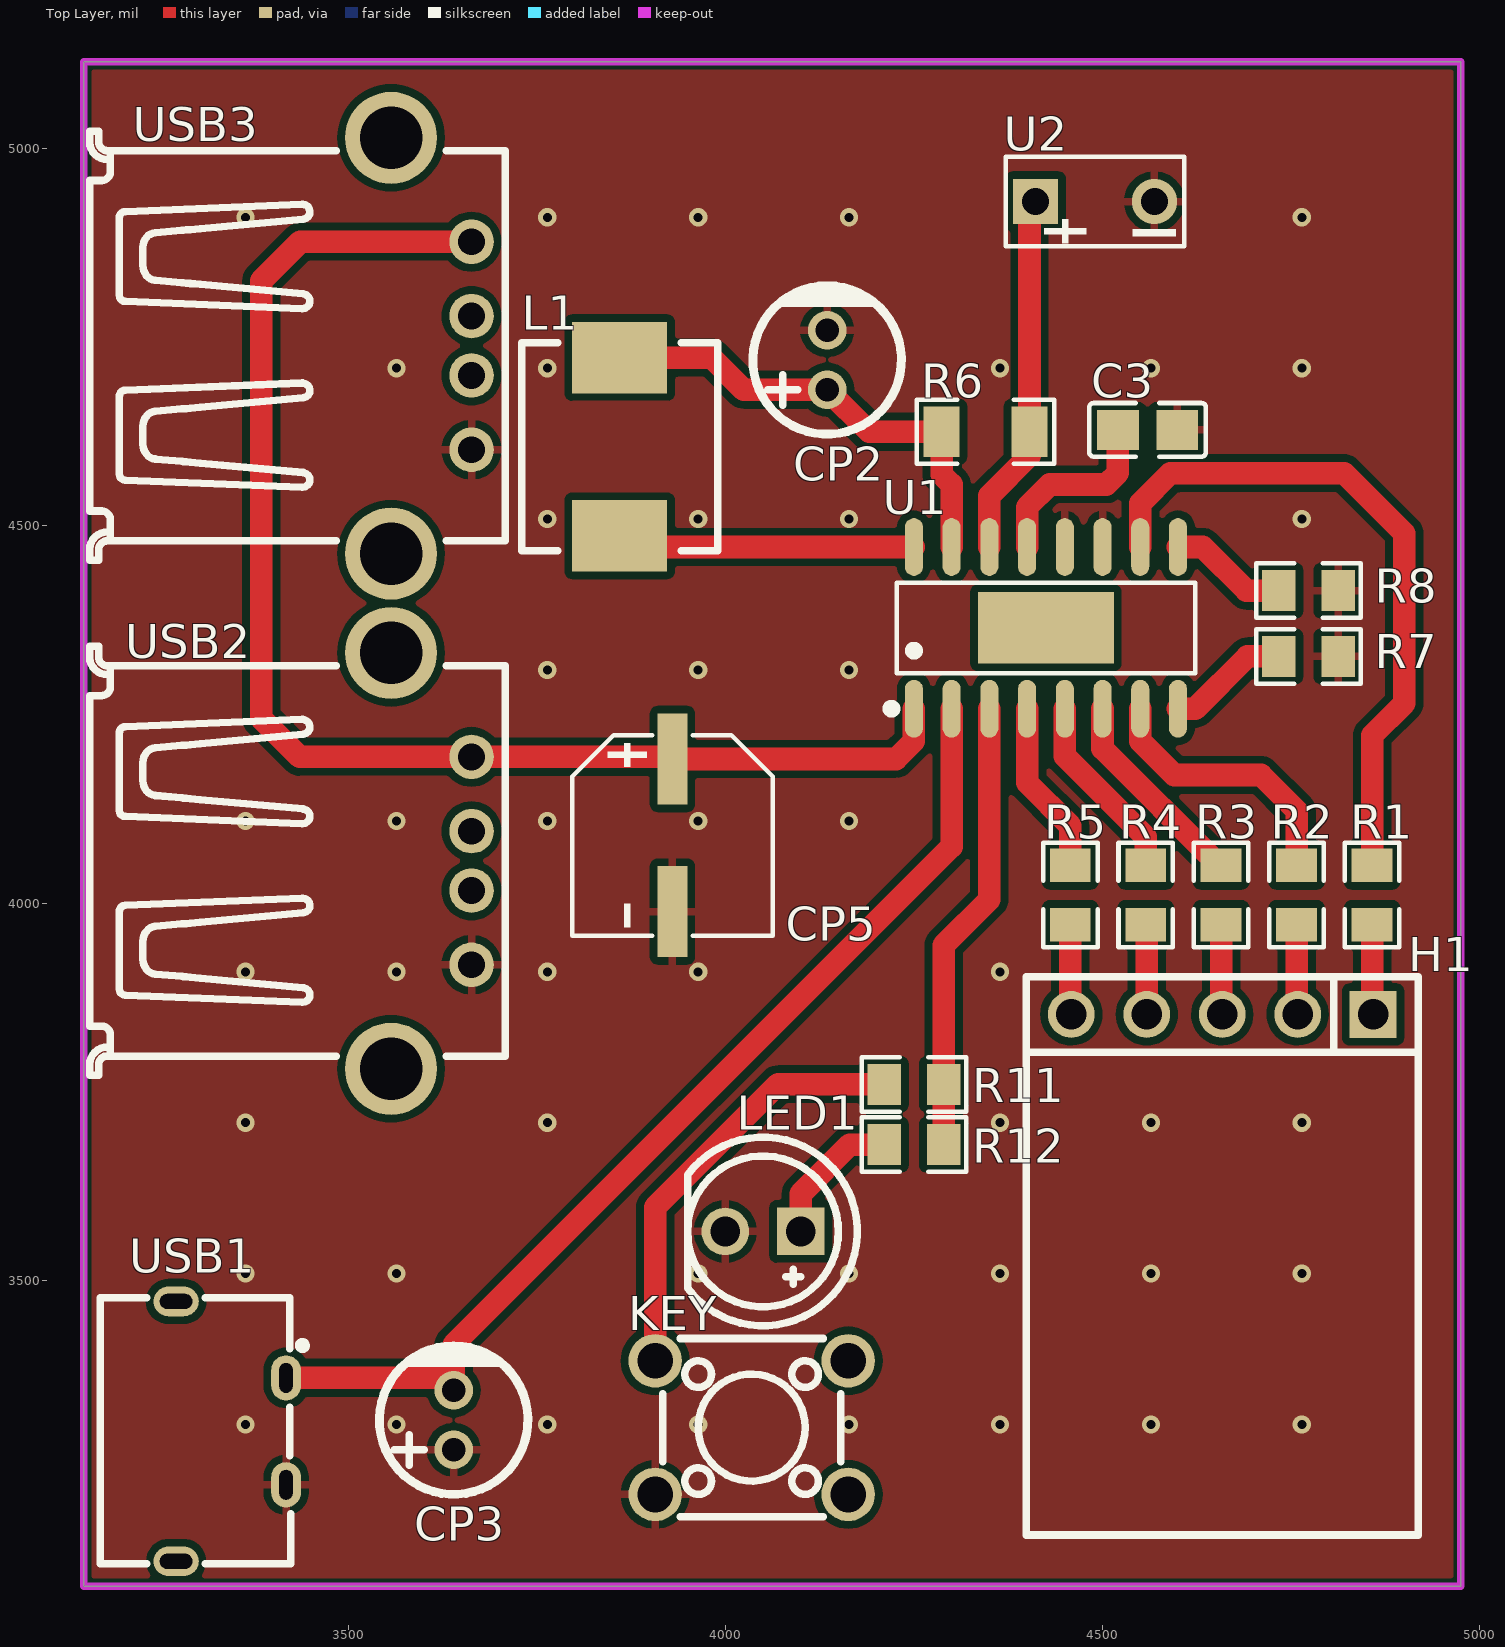
[diagram p0: Top Layer view]
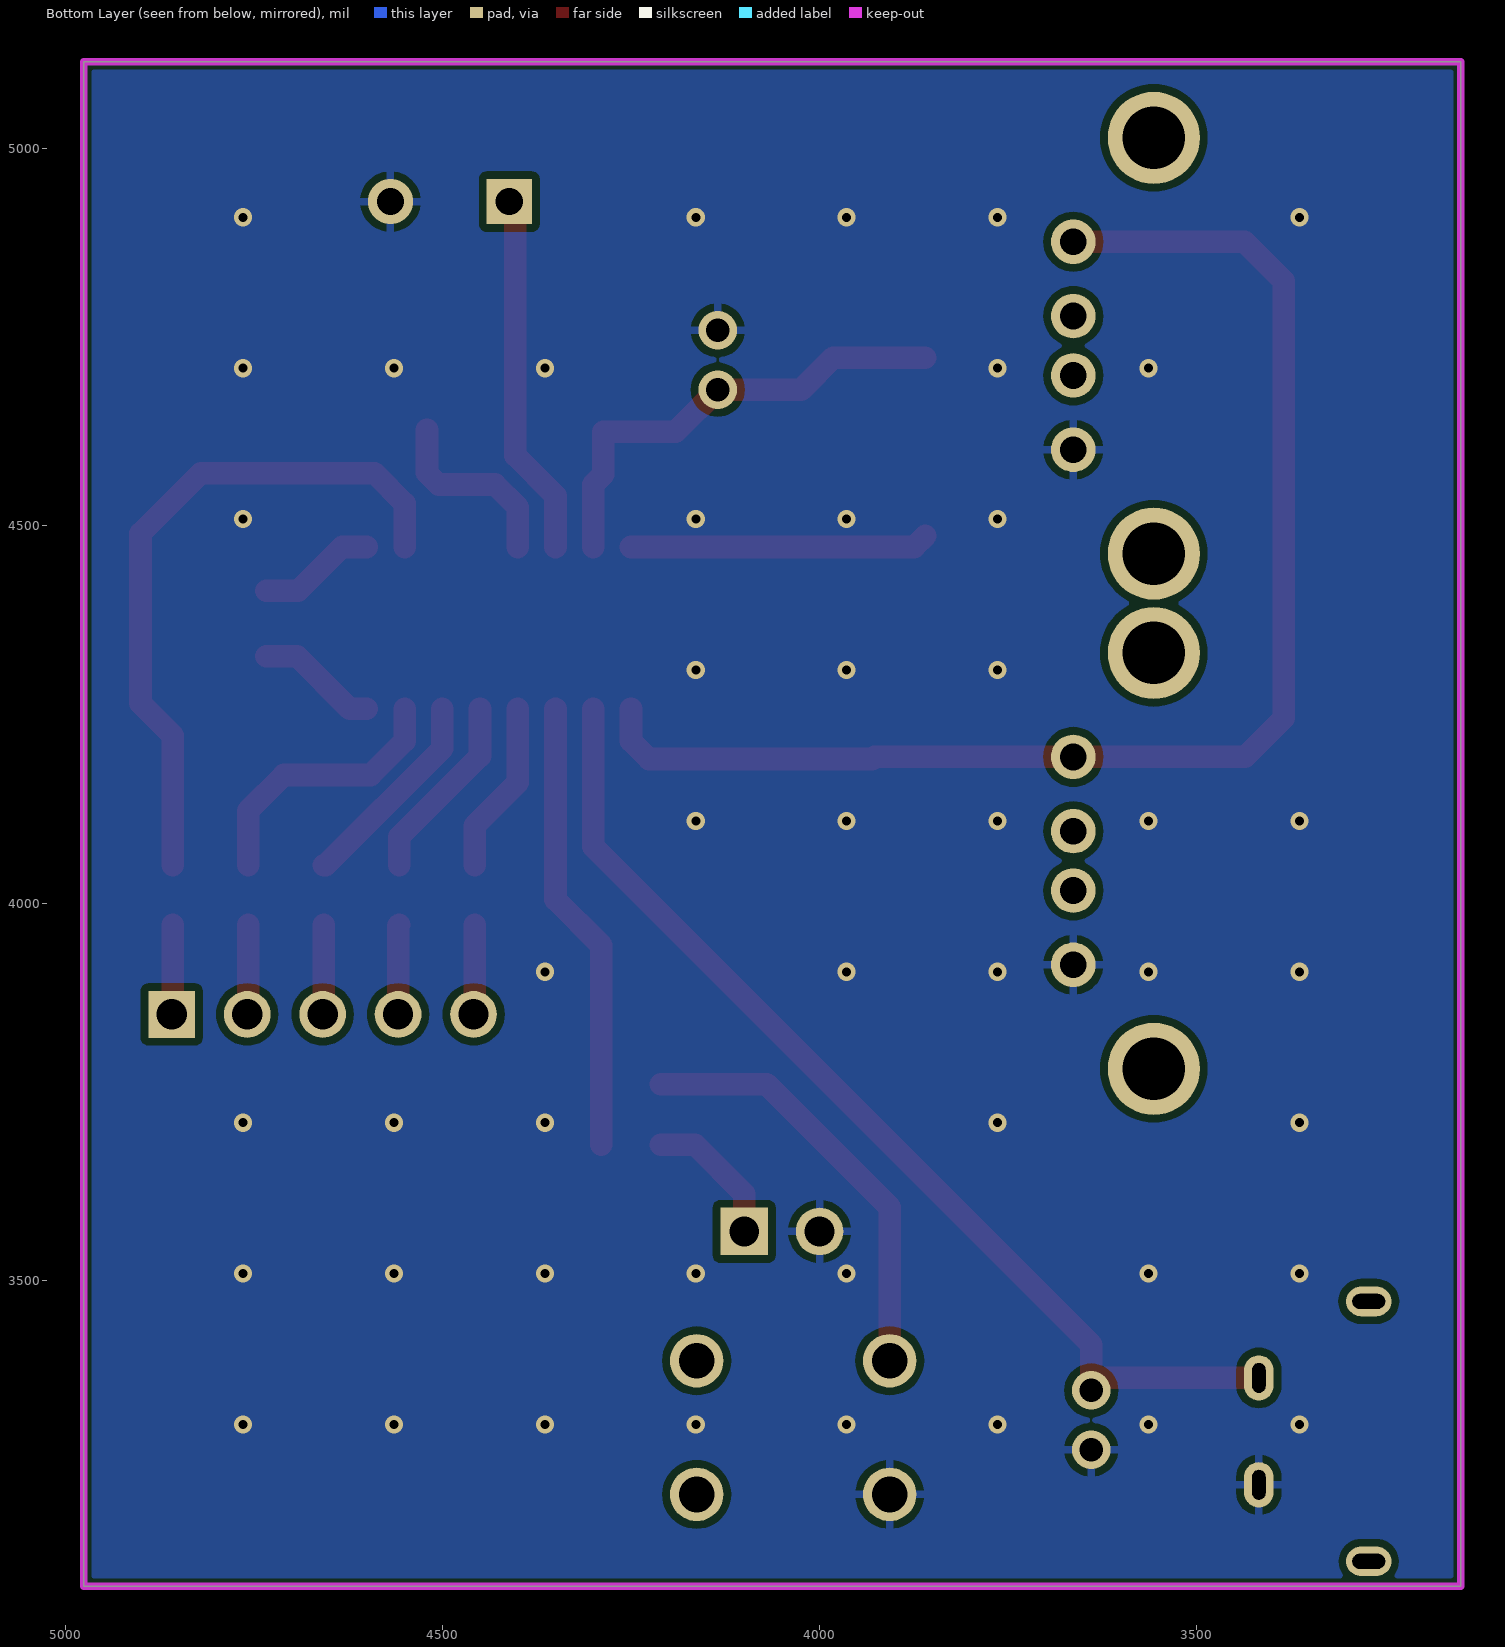
[diagram p1: Bottom Layer view, seen from below]
# Altium PCB MISC51911.pcbdoc
Units mil, origin at the board's own origin, x right, y up, seen from the top; angles counter-clockwise.
Board outline 1825 x 2020 mil, 2 copper layers (Top Layer, Bottom Layer), stack 62.206 mil thick; 23 components, 22 nets, 76 pads, 47 vias.

## Layer stack, top to bottom
Top Solder Mask Layer: solder mask 0.394, Dk 3.3
Top Layer: signal copper 1.379
Dielectric1: surface 59.449, FR4, Dk 4.5
Bottom Layer: signal copper 1.378
Bottom Solder Mask Layer: solder mask 0.394, Dk 3.3

## Board outline
3150,5115 3150,3095 4975,3095 4975,5115

## Design rules (kind name [scope] priority, off if disabled: settings)
BoardOutlineClearance copperThickness2oz_1 [All] p2 off: genericclearance=7.99 ignorepadtopadclearanceinfootprint=FALSE except(0: Arc-SplitContinuation Track-SplitContinuation SMDPad-SplitContinuation THPad-SplitContinuation Via-SplitContinuation Fill-SplitContinuation Region-SplitContinuation Poly-SplitContinuation Text-SplitContinuation Hole-SplitContinuation; 5.98: Arc-CutoutEdge SMDPad-CutoutEdge THPad-CutoutEdge Via-CutoutEdge Fill-CutoutEdge Region-CutoutEdge Text-CutoutEdge; 6.93: Hole-OutlineEdge Hole-CutoutEdge; 10: Poly-OutlineEdge Poly-CutoutEdge; 11.81: Arc-OutlineEdge Track-OutlineEdge SMDPad-OutlineEdge THPad-OutlineEdge Via-OutlineEdge Fill-OutlineEdge Region-OutlineEdge Text-OutlineEdge Track-CutoutEdge)
BoardOutlineClearance copperThickness1oz_1 [All] p4: genericclearance=4.02 ignorepadtopadclearanceinfootprint=FALSE except(0: Arc-SplitContinuation Track-SplitContinuation SMDPad-SplitContinuation THPad-SplitContinuation Via-SplitContinuation Fill-SplitContinuation Region-SplitContinuation Poly-SplitContinuation Text-SplitContinuation Hole-SplitContinuation; 6: SMDPad-CutoutEdge THPad-CutoutEdge Via-CutoutEdge Fill-CutoutEdge Region-CutoutEdge Text-CutoutEdge; 6.93: Hole-OutlineEdge Hole-CutoutEdge; 10: Poly-OutlineEdge Poly-CutoutEdge; 11.8: Arc-OutlineEdge Track-OutlineEdge SMDPad-OutlineEdge THPad-OutlineEdge Via-OutlineEdge Fill-OutlineEdge Region-OutlineEdge Text-OutlineEdge; 11.81: Arc-CutoutEdge Track-CutoutEdge)
Clearance copperThickness2oz [All] p1 off: gap=7.99 ignorepadtopadclearanceinfootprint=FALSE except(5.98: SMDPad-Track SMDPad-SMDPad THPad-Track SMDPad-THPad THPad-THPad Track-Via SMDPad-Via THPad-Via Via-Via Fill-Track Region-Track Fill-SMDPad Region-SMDPad Fill-THPad Region-THPad Fill-Via Region-Via Fill-Fill Fill-Region Region-Region Arc-Track Arc-SMDPad Arc-THPad Arc-Via Fill-Arc Region-Arc Arc-Arc Text-Track SMDPad-Text Text-THPad Text-Via Fill-Text Region-Text Arc-Text Text-Text; 6.93: Hole-Track Hole-SMDPad Hole-THPad Hole-Via Fill-Hole Region-Hole Hole-Arc Hole-Text; 10: Poly-Track Poly-SMDPad Poly-THPad Poly-Via Poly-Fill Poly-Region Poly-Poly Poly-Arc Poly-Text Poly-Hole)
Clearance copperThickness1oz [All] p3: gap=4.02 ignorepadtopadclearanceinfootprint=FALSE except(5.98: SMDPad-Track SMDPad-SMDPad THPad-Track SMDPad-THPad THPad-THPad Track-Via SMDPad-Via THPad-Via Via-Via Fill-Track Region-Track Fill-SMDPad Region-SMDPad Fill-THPad Region-THPad Fill-Via Region-Via Fill-Fill Fill-Region Region-Region; 6: Arc-Track Arc-SMDPad Arc-THPad Arc-Via Fill-Arc Region-Arc Arc-Arc Text-Track SMDPad-Text Text-THPad Text-Via Fill-Text Region-Text Arc-Text Text-Text; 6.93: Hole-Track Hole-SMDPad Hole-THPad Hole-Via Fill-Hole Region-Hole Hole-Arc Hole-Text; 10: Poly-Track Poly-SMDPad Poly-THPad Poly-Via Poly-Fill Poly-Region Poly-Poly Poly-Arc Poly-Text Poly-Hole)
DiffPairsRouting differentialPair [All] p1: maxlimit=6 minlimit=6 mostfreqgap=6 toplayer_minwidth=5 toplayer_prefwidth=10 toplayer_maxwidth=100 toplayer_mingap=6 toplayer_prefgap=6 toplayer_maxgap=6 bottomlayer_minwidth=5 bottomlayer_prefwidth=10 bottomlayer_maxwidth=100 bottomlayer_mingap=6 bottomlayer_prefgap=6 bottomlayer_maxgap=6 maxuncoupledlength=10
HoleToHoleClearance otherClearance [All] p1: gap=11.81 allowstackedmicrovias=TRUE
Length netLength [All] p1: minlimit=0 maxlimit=0
MatchedLengths netLengthTolerance [All] p1: tolerance=1000
PasteMaskExpansion pasteMaskExpansion [All] p1: expansion=0
PlaneConnect innerPlane [All] p1: planeconnectstyle=Relief reliefexpansion=20 reliefentries=4 reliefconductorwidth=10 reliefairgap=10
PolygonConnect copperRegion [(InNet('GND'))] p1: connectstyle=Relief reliefconductorwidth=10 reliefentries=4 polygonreliefangle="90 Angle" airgapwidth=10 via.connectstyle=Relief via.reliefconductorwidth=10 via.reliefentries=4 via.polygonreliefangle="90 Angle" via.airgapwidth=10
RoutingVias viaSize [All] p1: holewidth=12.01 width=24.02 viastyle="Through Hole" minholewidth=11.81 minwidth=19.68 maxholewidth=248.03 maxwidth=393.7
SolderMaskExpansion solderMaskExpansion [IsVia] p1: expansion=-1000 istentingtop=TRUE
SolderMaskExpansion solderMaskExpansion [All] p2: expansion=2 istentingtop=FALSE
Width copperThickness2oz_2 [All] p1 off: maxlimit=100 minlimit=8 preferedwidth=10
Width copperThickness1oz_2 [All] p2: maxlimit=100 minlimit=5 preferedwidth=10

## Components (designator, comment, footprint, x,y, rotation, side; value= is the part's Value field where it differs from the comment)
C3 "2.2uF" C0805 4559.68,4627.42 r180 top
CP2 "RT1_10uF/50V" CAP-TH_BD5.0-P2.00-D0.8-FD 4135,4720 r90 top
CP3 "RT1_10uF/50V" CAP-TH_BD5.0-P2.00-D0.8-FD 3640,3315 r90 top
CP5 "47uF/50V" CAP-SMD_BD6.3-L6.6-W6.6-LS7.0-FD 3930,4090 r270 top
H1 "" HDR-TH_5P-P2.54-V-F 4658.64,3852.66 r180 top
KEY "" SW-TH_4P-L6.0-W6.0-P4.50-LS6.5 4035,3305 r0 top
L1 "1uH" IND-SMD_L7.0-W6.6 3860,4605 r270 top
LED1 "" LED-TH_5mm 4050,3565 r180 top
R1 "510R" R0805 4857.27,4010.93 r270 top
R2 "510R" R0805 4757.27,4010.93 r270 top
R3 "510R" R0805 4657.27,4010.93 r270 top
R4 "510R" R0805 4557.27,4010.93 r270 top
R5 "510R" R0805 4457.27,4010.93 r270 top
R6 "合金电阻,0.01R" R1206 4345,4625 r180 top
R7 "15K" R0805 4772.93,4327.16 r0 top
R8 "1K" R0805 4772.93,4414.26 r0 top
R11 "10K" R0805 4250,3760 r180 top
R12 "20R" R0805 4250,3680 r180 top
U1 "IP5506-BZ-188" ESOP-16_L9.9-W3.9-P1.27-LS6.0-BL-EP 4425,4365 r0 top
U2 "电池盒接口" TH_C9900019910 4490,4930 r0 top
USB1 "KH-TYPE-C-2P" USB-SMD_KH-TYPE-C-2P 3345,3300 r270 top
USB2 "" "USB_ Type-A" 3448.74,4056.78 r270 top
USB3 "" "USB_ Type-A" 3448.74,4739.5 r270 top

## Footprints (in the part's own frame and the unit in brackets; to place one, negate y for a bottom-side part, rotate by r counter-clockwise, add the part's x,y. Pads: shape width x height; smd on the part's side, far side on the other; paste and mask are expansions set on the pad)
C0805 [mm]
  rect 1.41x1.35 smd paste-100 mask+0.051: 1(-1,0) 2(1,0)
  silkscreen extent -1.96,-0.9 1.96,0.9
CAP-SMD_BD6.3-L6.6-W6.6-LS7.0-FD [mm]
  rect 3.06x1 smd: 1(-2.57,0) 2(2.57,0)
  silkscreen extent -3.38,-3.38 3.38,3.38
CAP-TH_BD5.0-P2.00-D0.8-FD [mm]
  round 1.3 hole 0.8: 1(-1,0) 2(1,0)
  silkscreen extent -2.5,-2.5 2.5,2.5
ESOP-16_L9.9-W3.9-P1.27-LS6.0-BL-EP [mm]
  oval 0.609x1.944 smd: 1(-4.445,-2.722) 2(-3.175,-2.722) 3(-1.905,-2.722) 4(-0.635,-2.722) 5(0.635,-2.722) 6(1.905,-2.722) 7(3.175,-2.722) 8(4.445,-2.722) 9(4.445,2.722) 10(3.175,2.722) 11(1.905,2.722) 12(0.635,2.722) 13(-0.635,2.722) 14(-1.905,2.722) 15(-3.175,2.722) 16(-4.445,2.722)
  rect 4.57x2.41 smd: 17(0,0)
  silkscreen extent -5.35,-2.87 5.03,1.52
HDR-TH_5P-P2.54-V-F [mil]
  rect 62x62 hole 40.16: 1(-200,0)
  round 62 hole 40.16: 2(-100,0) 3(0,0) 4(100,0) 5(200,0)
  silkscreen extent -260,-50 260,50
IND-SMD_L7.0-W6.6 [mm]
  rect 2.4x3.2 smd: 1(-3,0) 2(3,0)
  silkscreen extent -3.5,-3.3 3.5,3.3
LED-TH_5mm [mm]
  rect 1.6x1.6 hole 1 paste+0 mask+0.051: 1(-1.27,0)
  round 1.6 hole 1 paste+0 mask+0.051: 2(1.27,0)
  silkscreen extent -3.17,-3.17 2.54,3.17
R0805 [mm]
  rect 1.133x1.377 smd paste-100 mask+0.051: 1(-1,0) 2(1,0)
  silkscreen extent -1.76,-0.92 1.76,0.92
R1206 [mil]
  rect 47.54x66.97 smd paste-3937.01 mask+2: 1(-58.22,0) 2(58.22,0)
  silkscreen extent -91,-42 91,42
SW-TH_4P-L6.0-W6.0-P4.50-LS6.5 [mm]
  round 1.8 hole 1.2: 1(-3.25,2.25) 2(3.25,2.25) 3(-3.25,-2.25) 4(3.25,-2.25)
  silkscreen extent -3,-3 3,3
TH_C9900019910 [mil]
  rect 60x60 hole 36 paste+0 mask+1.97: 1(-78.74,0)
  round 60 hole 36 paste+0 mask+1.97: 2(78.74,0)
  silkscreen extent -118,-59 118,59
USB-SMD_KH-TYPE-C-2P [mm]
  oval 1.524x1 hole 0.45 slot 1 at 0 deg paste+0 mask+0.05: 1(-1.8,1.85) 2(1.8,1.85)
  oval 1x1.524 hole 0.5 slot 1.1 at 90 deg paste+0 mask+0.05: 3(4.375,-1.85) 4(-4.375,-1.85)
  silkscreen extent -4.5,-4.41 4.46,2.53
"USB_ Type-A" [mm]
  round 1.5 hole 0.9 copper offset 0,0 paste+0 mask+0.051: 1(-3.484,5.461) 4(3.516,5.461)
  round 1.5 hole 0.9 paste+0 mask+0.051: 2(-0.984,5.461) 3(1.016,5.461)
  round 3.1 hole 2.1 paste+0 mask+0.051: SH1(7.016,2.751) SH2(-6.984,2.751)
  silkscreen extent -7.2,-7.4 7.24,6.6

## Via types
v1: diameter 24.02, hole 12, Top Layer to Bottom Layer, 47 vias

## Nets (pads, with @x,y where several pads share a name; then routed paths per layer and width w, separated by ;. In a path a pad name is that pad's centre, name@x,y a point inside that pad or via, vN(x,y) a via of type N, cw(c..) or ccw(c..) an arc to the next point about the centre after c; other vN are vias at no path point)
$1N4: CP5.1 U1.1 USB2.1 USB3.1 | length 1820.1
  Top Layer w30: USB3.1 3436.67,4876.67 3385,4825 3385,4245 3436.05,4193.95 USB2.1 3927.23,4193.95 CP5.1 4226.18,4191.18 4250,4215 U1.1
$1N6: CP3.2 U1.2 USB1.1 | length 1405.8
  Top Layer w30: USB1.1 3623.5,3370.87 CP3.2 3640,3415 4300,4075 U1.2
$1N9: R6.1 U1.14 U2.1 | length 483.2
  Top Layer w30: U1.14 4350,4540 4403.22,4593.22 R6.1 4403.22,4921.96 U2.1
$1N11: CP2.1 L1.1 R6.2 U1.15 | length 625.7
  Top Layer w30: L1.1 3981.89,4723.11 4024.37,4680.63 CP2.1 4190.63,4625 R6.2 4286.78,4568.22 4300,4555 U1.15
$1N12: L1.2 U1.16 | length 396.1
  Top Layer w30: L1.2 3874.71,4472.18 U1.16
$1N14: C3.2 U1.13 | length 249
  Top Layer w30: U1.13 4400,4525 4430,4555 4505,4555 4520.31,4570.31 C3.2
$1N16: R1.1 U1.10 | length 914.9
  Top Layer w30: U1.10 4550,4530 4590,4570 4820,4570 4900,4490 4900,4265 4857.27,4222.27 R1.1
$1N17: R2.1 U1.7 | length 360.7
  Top Layer w30: U1.7 4550,4215 4595,4170 4710,4170 4757.27,4122.73 R2.1
$1N18: R3.1 U1.6 | length 274.2
  Top Layer w30: U1.6 4500,4205 4654.7,4050.3 R3.1
$1N19: R4.1 U1.5 | length 252
  Top Layer w30: U1.5 4450,4195 4557.27,4087.73 R4.1
$1N20: R5.1 U1.4 | length 231.2
  Top Layer w30: U1.4 4400,4160 4457.27,4102.73 R5.1
$1N21: H1.1 R1.2 | length 119.5
  Top Layer w30: R1.2 4857.27,3854.03 H1.1
$1N22: H1.2 R2.2 | length 119.5
  Top Layer w30: R2.2 4757.27,3854.03 H1.2
$1N23: H1.3 R3.2 | length 119.5
  Top Layer w30: R3.2 4657.27,3854.03 H1.3
$1N24: H1.4 R4.2 | length 119.5
  Top Layer w30: R4.2 4558.64,3970.2 H1.4
$1N25: H1.5 R5.2 | length 119.5
  Top Layer w30: R5.2 4457.27,3854.03 H1.5
$1N27: R7.1 U1.8 | length 162.3
  Top Layer w30: U1.8 4622.82,4257.82 4692.16,4327.16 R7.1
$1N28: R8.1 U1.9 | length 157.5
  Top Layer w30: U1.9 4632.82,4472.18 4690.74,4414.26 R8.1
$1N31: KEY.1 R11.2 | length 574.5
  Top Layer w30: KEY.1 3907.05,3597.05 4070,3760 R11.2
$1N32: LED1.1 R12.2 | length 187.6
  Top Layer w30: LED1.1 4100,3615 4165,3680 R12.2
$1N33: R11.1 R12.1 U1.3 | length 602.9
  Top Layer w30: R12.1 R11.1 4289.37,3944.37 4350,4005 U1.3
GND: C3.1 CP2.2 CP3.1 CP5.2 KEY.3 LED1.2 R7.2 R8.2 U1.11 U1.12 U2.2 USB1.2 USB2.4 USB3.4
  other v1: 3364.1,3309.1 3564.1,3309.1 3764.1,3309.1 3964.1,3309.1 4164.1,3309.1 4364.1,3309.1 4564.1,3309.1 4764.1,3309.1 3364.1,3509.1 3564.1,3509.1 3964.1,3509.1 4164.1,3509.1 4364.1,3509.1 4564.1,3509.1 4764.1,3509.1 3364.1,3709.1 3764.1,3709.1 4364.1,3709.1 4564.1,3709.1 4764.1,3709.1 3364.1,3909.1 3564.1,3909.1 3764.1,3909.1 3964.1,3909.1 4364.1,3909.1 3364.1,4109.1 3564.1,4109.1 3764.1,4109.1 3964.1,4109.1 4164.1,4109.1 3764.1,4309.1 3964.1,4309.1 4164.1,4309.1 3764.1,4509.1 3964.1,4509.1 4164.1,4509.1 4764.1,4509.1 3564.1,4709.1 3764.1,4709.1 4364.1,4709.1 4564.1,4709.1 4764.1,4709.1 3364.1,4909.1 3764.1,4909.1 3964.1,4909.1 4164.1,4909.1 4764.1,4909.1
pads on no net: KEY.2 KEY.4 U1.17 USB1.3 USB1.4 USB2.2 USB2.3 USB2.SH1 USB2.SH2 USB3.2 USB3.3 USB3.SH1 USB3.SH2

## Polygon pours and split planes (outlines as drawn)
GND on Top Layer (solid, remove dead copper, pour order 0): 3000,5160 3000,3000 5205,3000 5205,5160
GND on Bottom Layer (solid, remove dead copper, pour order 2): 3035,5190 3035,3005 5260,3005 5260,5190

## Keep-outs
Board Outline Layer:
  the board outline again, w10

## Silkscreen, mask and mechanical layers (free items; w line width, h text height)
Top Silkscreen Layer:
  lines w10: 4398.79,3162.66 4398.79,3902.66 4918.48,3902.66 4918.48,3162.66 4398.79,3162.66